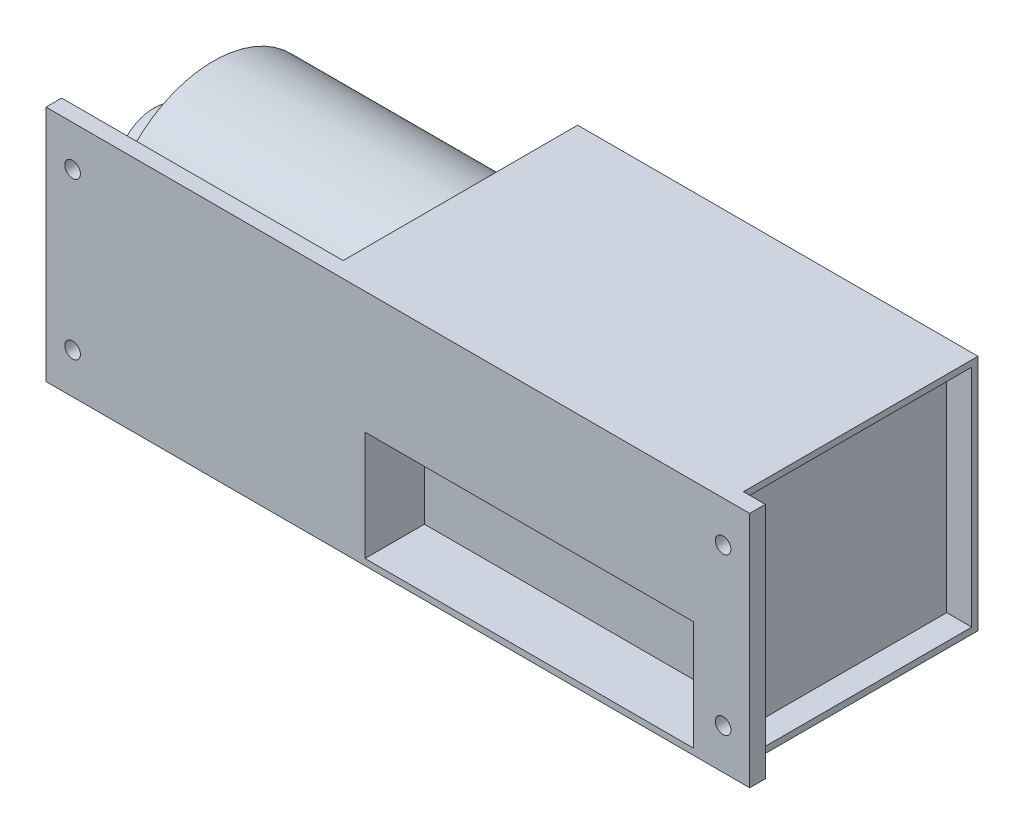
from build123d import *

# Parameters (mm, degrees)
SKETCH_1_W          = 225
SKETCH_1_H          = 76
EXTRUDE_1_DEPTH     = 80
SKETCH_2_W          = 75
SKETCH_2_H          = 76
CUT_EXTRUDE_1_DEPTH = 90
SKETCH_3_W          = 75
SKETCH_3_H          = 76
CUT_EXTRUDE_2_DEPTH = 15
SKETCH_4_R          = 2.5
CUT_EXTRUDE_3_DEPTH = 15
SKETCH_5_R          = 35
EXTRUDE_2_DEPTH     = 79
SKETCH_6_R          = 12.5
EXTRUDE_3_DEPTH     = 19
SKETCH_7_W          = 105
SKETCH_7_H          = 35
CUT_EXTRUDE_4_DEPTH = 19
EXTRUDE_4_DEPTH     = 8


with BuildPart() as part:
    # 草图1 → 凸台-拉伸1 (new body)
    with BuildSketch(Plane.XY):
        Rectangle(SKETCH_1_W, SKETCH_1_H)
    extrude(amount=EXTRUDE_1_DEPTH)

    # 草图2 → 切除-拉伸1 (cut)
    with BuildSketch(Plane.ZY.offset(112.5)):
        with Locations((37.5, 0)):
            Rectangle(SKETCH_2_W, SKETCH_2_H)
    extrude(amount=-CUT_EXTRUDE_1_DEPTH, mode=Mode.SUBTRACT)

    # 草图3 → 切除-拉伸2 (cut)
    with BuildSketch(Plane(origin=(112.5, 0, 0), x_dir=(0, 0, -1), z_dir=(1, 0, 0))):
        with Locations((-37.5, 0)):
            Rectangle(SKETCH_3_W, SKETCH_3_H)
    extrude(amount=-CUT_EXTRUDE_2_DEPTH, mode=Mode.SUBTRACT)

    # 草图4 → 切除-拉伸3 (cut)
    with BuildSketch(Plane(origin=(0, 0, 75), x_dir=(-1, 0, 0), z_dir=(0, 0, -1))):
        with Locations((104, -25)):
            Circle(SKETCH_4_R)
        with Locations((104, 25)):
            Circle(SKETCH_4_R)
        with Locations((-104, -25)):
            Circle(SKETCH_4_R)
        with Locations((-104, 25)):
            Circle(SKETCH_4_R)
    extrude(amount=-CUT_EXTRUDE_3_DEPTH, mode=Mode.SUBTRACT)

    # 草图5 → 凸台-拉伸2 (add)
    with BuildSketch(Plane.ZY.offset(22.5)):
        with Locations(Location((37.5, 0, 0), (0, 0, 180))):
            Circle(SKETCH_5_R)
    extrude(amount=EXTRUDE_2_DEPTH)

    # 草图6 → 凸台-拉伸3 (add)
    with BuildSketch(Plane.ZY.offset(101.5)):
        with Locations((37.5, 0)):
            Circle(SKETCH_6_R)
    extrude(amount=EXTRUDE_3_DEPTH)

    # 草图7 → 切除-拉伸4 (cut)
    with BuildSketch(Plane.XY.offset(80)):
        with Locations((42, -18.5)):
            Rectangle(SKETCH_7_W, SKETCH_7_H)
    extrude(amount=-CUT_EXTRUDE_4_DEPTH, mode=Mode.SUBTRACT)

    # 草图8 → 凸台-拉伸4 (add)
    with BuildSketch(Plane(origin=(97.5, 0, 0), x_dir=(0, 0, -1), z_dir=(1, 0, 0))):
        Polygon((-75, 38), (0, 38), (0, -38), (-75, -38), (-75, -36), (-2, -36), (-2, 36), (-75, 36), align=None)
    extrude(amount=EXTRUDE_4_DEPTH)


solid = part.part
